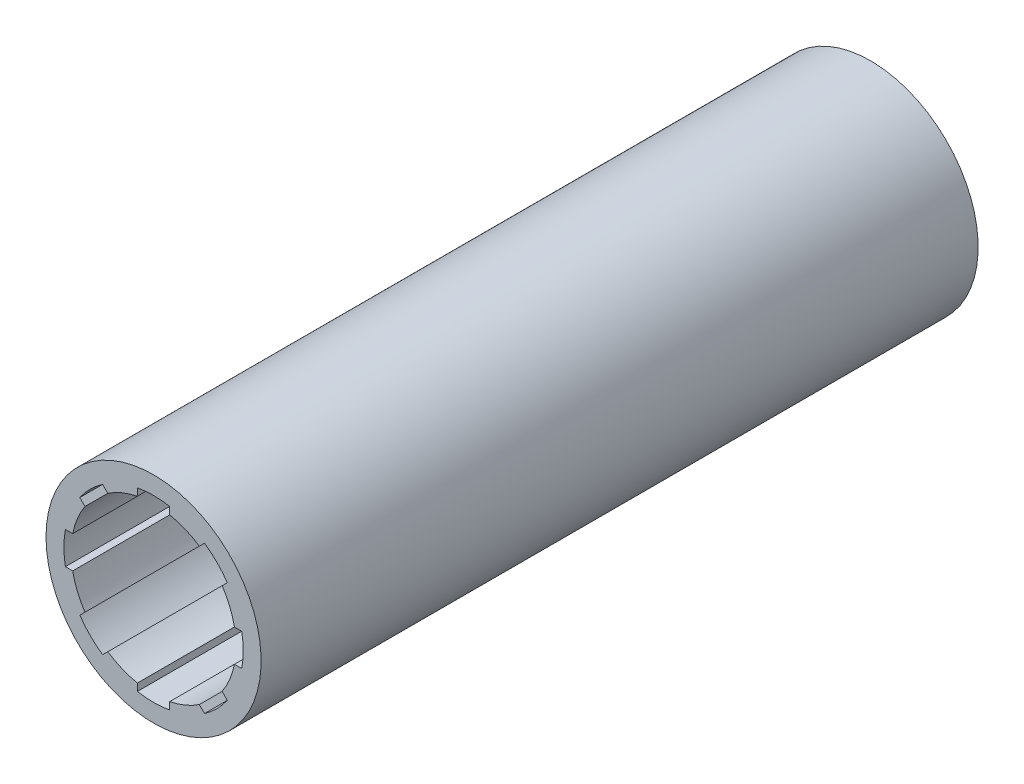
SolidWorks part; units mm, degrees
ref_plane "前视基准面" through (0, 0, 0) normal (0, 0, 1) x (1, 0, 0)
ref_plane "上视基准面" through (0, 0, 0) normal (0, 1, 0) x (1, 0, 0)
ref_plane "右视基准面" through (0, 0, 0) normal (1, 0, 0) x (0, 0, -1)
sketch "草图1" plane through (0, 0, 0) normal (0, 0, 1) x (1, 0, 0)
  circle A0 centre (0, 0) radius 30
  dimension "D1" = 60
extrude "凸台-拉伸1" add sketch "草图1" along normal mid plane 200
sketch "草图2" plane through (0, 0, 100) normal (0, 0, 1) x (1, 0, 0)
  line L0 (-4.5, 24.5917) -> (-4.5, 22.5555)
  line L2 (4.5, 22.5555) -> (4.5, 24.5917)
  line L4 (0, 0) -> (0, 25) construction
  line L5 (14.207, 20.5709) -> (12.7672, 19.1311)
  line L6 (19.1311, 12.7672) -> (20.5709, 14.207)
  line L7 (24.5917, 4.5) -> (22.5555, 4.5)
  line L8 (22.5555, -4.5) -> (24.5917, -4.5)
  line L9 (20.5709, -14.207) -> (19.1311, -12.7672)
  line L10 (12.7672, -19.1311) -> (14.207, -20.5709)
  line L11 (4.5, -24.5917) -> (4.5, -22.5555)
  line L12 (-4.5, -22.5555) -> (-4.5, -24.5917)
  line L13 (-14.207, -20.5709) -> (-12.7672, -19.1311)
  line L14 (-19.1311, -12.7672) -> (-20.5709, -14.207)
  line L15 (-24.5917, -4.5) -> (-22.5555, -4.5)
  line L16 (-22.5555, 4.5) -> (-24.5917, 4.5)
  line L17 (-20.5709, 14.207) -> (-19.1311, 12.7672)
  line L18 (-12.7672, 19.1311) -> (-14.207, 20.5709)
  arc A0 (-4.5, 22.5555) -> (-12.7672, 19.1311) centre (0, 0) ccw
  arc A1 (4.5, 24.5917) -> (-4.5, 24.5917) centre (0, 0) ccw
  arc A2 (20.5709, 14.207) -> (14.207, 20.5709) centre (0, 0) ccw
  arc A3 (24.5917, -4.5) -> (24.5917, 4.5) centre (0, 0) ccw
  arc A4 (14.207, -20.5709) -> (20.5709, -14.207) centre (0, 0) ccw
  arc A5 (-4.5, -24.5917) -> (4.5, -24.5917) centre (0, 0) ccw
  arc A6 (-20.5709, -14.207) -> (-14.207, -20.5709) centre (0, 0) ccw
  arc A7 (-24.5917, 4.5) -> (-24.5917, -4.5) centre (0, 0) ccw
  arc A8 (-14.207, 20.5709) -> (-20.5709, 14.207) centre (0, 0) ccw
  arc A9 (-19.1311, 12.7672) -> (-22.5555, 4.5) centre (0, 0) ccw
  arc A10 (-22.5555, -4.5) -> (-19.1311, -12.7672) centre (0, 0) ccw
  arc A11 (-12.7672, -19.1311) -> (-4.5, -22.5555) centre (0, 0) ccw
  arc A12 (4.5, -22.5555) -> (12.7672, -19.1311) centre (0, 0) ccw
  arc A13 (19.1311, -12.7672) -> (22.5555, -4.5) centre (0, 0) ccw
  arc A14 (22.5555, 4.5) -> (19.1311, 12.7672) centre (0, 0) ccw
  arc A15 (12.7672, 19.1311) -> (4.5, 22.5555) centre (0, 0) ccw
  point P37 (0, 0)
  dimension "D1" = 46
  dimension "D2" = 50
  dimension "D3" = 9
  dimension "D4" = 8
extrude "切除-拉伸1" cut sketch "草图2" against normal blind 80
sketch "草图3" plane through (0, 0, -100) normal (0, 0, -1) x (-1, 0, 0)
  line L0 (-4, 22.6495) -> (-4, 20.6155)
  line L2 (4, 20.6155) -> (4, 22.6495)
  line L4 (0, 46.3047) -> (0, -43.702) construction
  line L5 (0, 55) -> (0, -55) construction
  line L6 (13.1872, 18.844) -> (11.749, 17.4058)
  line L7 (17.4058, 11.749) -> (18.844, 13.1872)
  line L8 (22.6495, 4) -> (20.6155, 4)
  line L9 (20.6155, -4) -> (22.6495, -4)
  line L10 (18.844, -13.1872) -> (17.4058, -11.749)
  line L11 (11.749, -17.4058) -> (13.1872, -18.844)
  line L12 (4, -22.6495) -> (4, -20.6155)
  line L13 (-4, -20.6155) -> (-4, -22.6495)
  line L14 (-13.1872, -18.844) -> (-11.749, -17.4058)
  line L15 (-17.4058, -11.749) -> (-18.844, -13.1872)
  line L16 (-22.6495, -4) -> (-20.6155, -4)
  line L17 (-20.6155, 4) -> (-22.6495, 4)
  line L18 (-18.844, 13.1872) -> (-17.4058, 11.749)
  line L19 (-11.749, 17.4058) -> (-13.1872, 18.844)
  arc A0 (-4, 20.6155) -> (-11.749, 17.4058) centre (0, 0) ccw
  arc A1 (4, 22.6495) -> (-4, 22.6495) centre (0, 0) ccw
  arc A2 (18.844, 13.1872) -> (13.1872, 18.844) centre (0, 0) ccw
  arc A3 (22.6495, -4) -> (22.6495, 4) centre (0, 0) ccw
  arc A4 (13.1872, -18.844) -> (18.844, -13.1872) centre (0, 0) ccw
  arc A5 (-4, -22.6495) -> (4, -22.6495) centre (0, 0) ccw
  arc A6 (-18.844, -13.1872) -> (-13.1872, -18.844) centre (0, 0) ccw
  arc A7 (-22.6495, 4) -> (-22.6495, -4) centre (0, 0) ccw
  arc A8 (-13.1872, 18.844) -> (-18.844, 13.1872) centre (0, 0) ccw
  arc A9 (-17.4058, 11.749) -> (-20.6155, 4) centre (0, 0) ccw
  arc A10 (-20.6155, -4) -> (-17.4058, -11.749) centre (0, 0) ccw
  arc A11 (-11.749, -17.4058) -> (-4, -20.6155) centre (0, 0) ccw
  arc A12 (4, -20.6155) -> (11.749, -17.4058) centre (0, 0) ccw
  arc A13 (17.4058, -11.749) -> (20.6155, -4) centre (0, 0) ccw
  arc A14 (20.6155, 4) -> (17.4058, 11.749) centre (0, 0) ccw
  arc A15 (11.749, 17.4058) -> (4, 20.6155) centre (0, 0) ccw
  point P40 (0, 0)
  dimension "D1" = 42
  dimension "D2" = 46
  dimension "D3" = 8
  dimension "D4" = 8
extrude "切除-拉伸2" cut sketch "草图3" against normal blind 80
